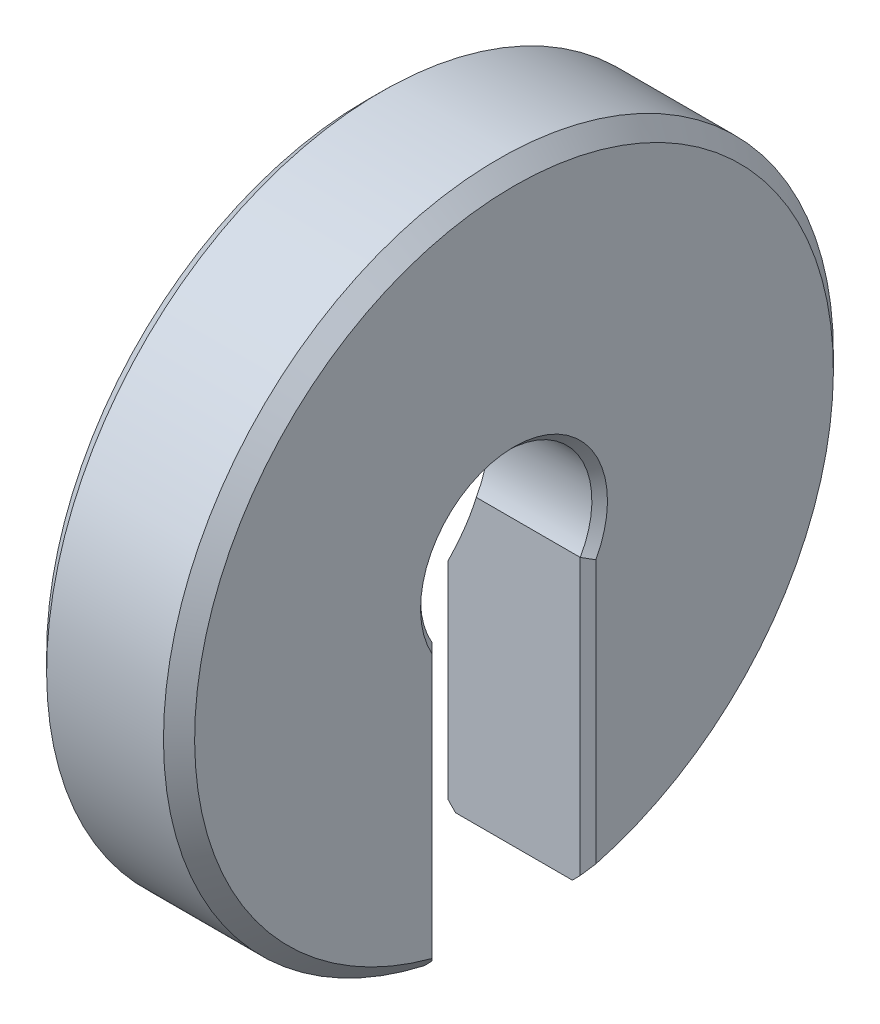
from build123d import *

# Parameters (mm, degrees)
CHAMFER1_SIZE      = 2
CUT_EXTRUDE2_DEPTH = 43
CHAMFER2_SIZE      = 1


with BuildPart() as part:
    # Sketch1 → Revolve1 (revolve)
    with BuildSketch(Plane.XY, mode=Mode.PRIVATE) as revolve1_sk:
        Polygon((-19, 19.05), (-19, 43), (0, 43), (0, 11), (-14.35, 11), align=None)
    revolve(revolve1_sk.sketch.rotate(Axis((-44.950542037, 0, 0), (1, 0, 0)), 90), axis=Axis((-44.950542037, 0, 0), (1, 0, 0)))

    # Chamfer1
    chamfer1_edges = [part.edges().sort_by_distance(p)[0] for p in [
        (-19, 0, -43),
        (0, 0, -43),
    ]]
    chamfer(chamfer1_edges, length=CHAMFER1_SIZE)

    # Sketch13 → Cut-Extrude2 (cut)
    with BuildSketch(Plane.ZY.offset(19)):
        Polygon((-9.5, 0), (-9.5, -65.513992054), (9.5, -73.697131866), (9.5, 0), align=None)
    extrude(amount=-CUT_EXTRUDE2_DEPTH, mode=Mode.SUBTRACT)

    # Chamfer2
    chamfer2_edges = [part.edges().sort_by_distance(p)[0] for p in [
        (-19, -28.198199933, -9.5),
        (-19, -28.198199933, 9.5),
        (0, -22.714737827, -9.5),
        (0, 11, 0),
        (0, -22.714737827, 9.5),
    ]]
    chamfer(chamfer2_edges, length=CHAMFER2_SIZE)


solid = part.part
